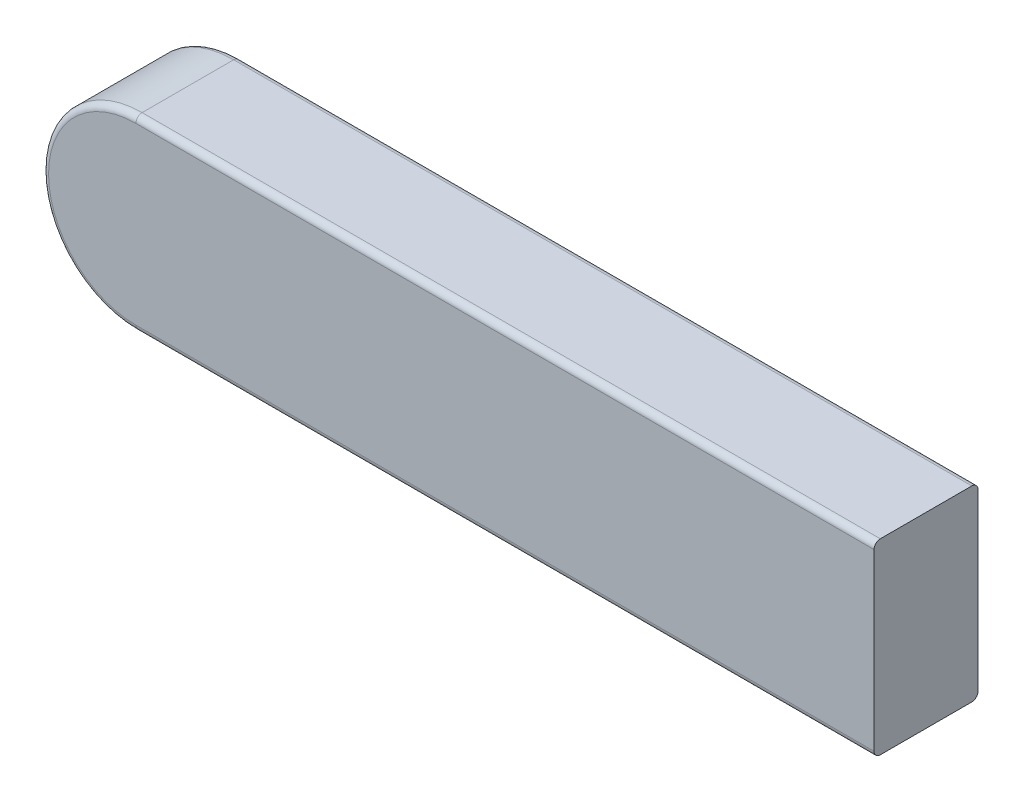
from build123d import *

# Parameters (mm, degrees)
BASE_EXTRUDE_DEPTH = 20
FILLET1_R          = 1.2


with BuildPart() as part:
    # Sketch1 → Base-Extrude (new body)
    with BuildSketch(Plane.XY):
        with BuildLine():
            Line((-9, 18), (133, 18))
            Line((133, 18), (133, -18))
            Line((133, -18), (-9, -18))
            ThreePointArc((-9, -18), (-27, 0), (-9, 18))
        make_face()
    extrude(amount=BASE_EXTRUDE_DEPTH)

    # Fillet1
    fillet1_edges = [part.edges().sort_by_distance(p)[0] for p in [
        (-27, 0, 20),
        (62, -18, 20),
        (62, -18, 0),
        (-27, 0, 0),
        (62, 18, 0),
        (62, 18, 20),
    ]]
    fillet(fillet1_edges, radius=FILLET1_R)


solid = part.part
